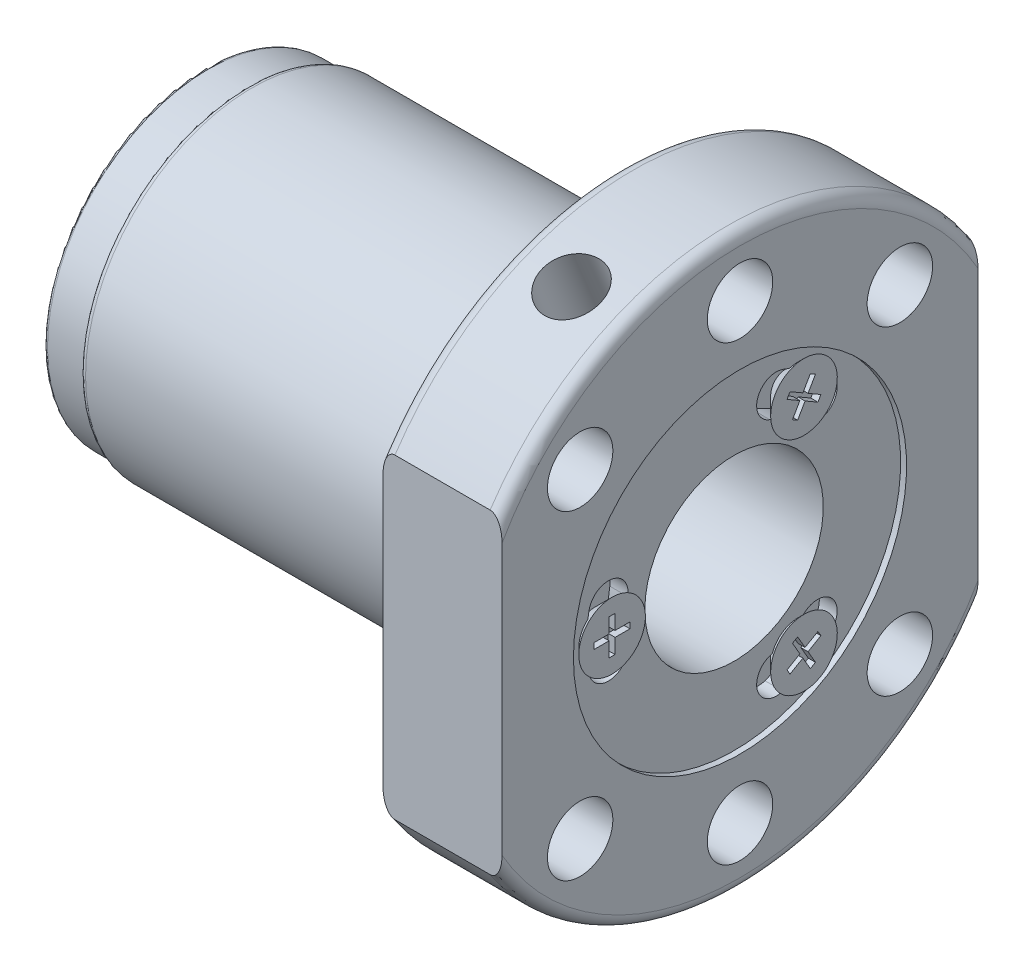
from build123d import *

# Parameters (mm, degrees)
SKETCH2_OUTSIDE_W   = 66.288
SKETCH2_OUTSIDE_H   = 66.288
SKETCH2_OUTSIDE_W_2 = 40
SKETCH2_OUTSIDE_H_2 = 48
CUT_EXTRUDE1_DEPTH  = 10
DIAMETERHOLE1_D     = 5.5
TAP1_REACH          = 66.874
TAP1_BORE_R         = 2.4585
CUT_EXTRUDE2_DEPTH  = 1.5
CUT_EXTRUDE3_DEPTH  = 0.6
CIRPATTERN1_COUNT   = 3


with BuildPart() as part:
    # Sketch1 → Revolve1 (revolve)
    with BuildSketch(Plane.XY, mode=Mode.PRIVATE) as revolve1_sk:
        with BuildLine():
            Line((10, 14), (9.5, 14))
            Line((9.5, 14), (9.5, 7.5))
            Line((9.5, 7.5), (-35, 7.5))
            Line((-35, 7.5), (-35, 13.2))
            ThreePointArc((-35, 13.2), (-34.912132034, 13.412132034), (-34.7, 13.5))
            Line((-34.7, 13.5), (-31.5, 13.5))
            ThreePointArc((-31.5, 13.5), (-31.353553391, 13.853553391), (-31, 14))
            Line((-31, 14), (0, 14))
            Line((0, 14), (0, 23))
            ThreePointArc((0, 23), (0.292893219, 23.707106781), (1, 24))
            Line((1, 24), (9, 24))
            ThreePointArc((9, 24), (9.707106781, 23.707106781), (10, 23))
            Line((10, 23), (10, 14))
        make_face()
    revolve(revolve1_sk.sketch.rotate(Axis((-37.257548112, 0, 0), (1, 0, 0)), 90), axis=Axis((-37.257548112, 0, 0), (1, 0, 0)))

    # Sketch2 outside → Cut-Extrude1 (cut)
    with BuildSketch(Plane(origin=(10, 0, 0), x_dir=(0, 0, -1), z_dir=(1, 0, 0))):
        Rectangle(SKETCH2_OUTSIDE_W, SKETCH2_OUTSIDE_H)
        Rectangle(SKETCH2_OUTSIDE_W_2, SKETCH2_OUTSIDE_H_2, mode=Mode.SUBTRACT)
    extrude(amount=-CUT_EXTRUDE1_DEPTH, mode=Mode.SUBTRACT)

    # DiameterHole1 (through all)
    with Locations(Plane(origin=(10, 0, 0), x_dir=(0, 0, -1), z_dir=(1, 0, 0))):
        with Locations((13.435028843, 13.435028843), (0, 19), (-13.435028843, 13.435028843), (-13.435028843, -13.435028843), (0, -19), (13.435028843, -13.435028843)):
            Hole(DIAMETERHOLE1_D / 2)

    # Tap1 bore → Tap1 (cut, up to next)
    with BuildSketch(Plane(origin=(0, 22.17310878, 9.184402377), x_dir=(1, 0, 0), z_dir=(0, 0.9238795325112865, 0.3826834323650906)), mode=Mode.PRIVATE) as tap1_sk1:
        with Locations((5, 0)):
            Circle(TAP1_BORE_R)
    tap1_tool1 = extrude(tap1_sk1.sketch, amount=-TAP1_REACH, mode=Mode.PRIVATE) & part.part
    add(tap1_tool1.solids().sort_by_distance((5, 22.173109, 9.184402))[0], mode=Mode.SUBTRACT)

    # Sketch7 → Cut-Extrude2 (cut)
    with BuildSketch(Plane(origin=(9.5, 0, 0), x_dir=(0, 0, -1), z_dir=(1, 0, 0))):
        with BuildLine():
            ThreePointArc((-12.183507635, 2.306976744), (-12.4, 0), (-12.183507635, -2.306976744))
            ThreePointArc((-12.183507635, -2.306976744), (-10.255338343, -3.621192548), (-8.941122539, -1.693023256))
            ThreePointArc((-8.941122539, -1.693023256), (-9.1, 0), (-8.941122539, 1.693023256))
            ThreePointArc((-8.941122539, 1.693023256), (-10.255338343, 3.621192548), (-12.183507635, 2.306976744))
        make_face()
        with BuildLine():
            ThreePointArc((8.089654284, 9.397738747), (6.2, 10.738715007), (4.093853351, 11.704715492))
            ThreePointArc((4.093853351, 11.704715492), (1.991624433, 10.691979804), (3.004360121, 8.589750885))
            ThreePointArc((3.004360121, 8.589750885), (4.55, 7.880831174), (5.936762418, 6.896727629))
            ThreePointArc((5.936762418, 6.896727629), (8.26371391, 7.070787255), (8.089654284, 9.397738747))
        make_face()
        with BuildLine():
            ThreePointArc((4.093853351, -11.704715492), (6.2, -10.738715007), (8.089654284, -9.397738747))
            ThreePointArc((8.089654284, -9.397738747), (8.26371391, -7.070787255), (5.936762418, -6.896727629))
            ThreePointArc((5.936762418, -6.896727629), (4.55, -7.880831174), (3.004360121, -8.589750885))
            ThreePointArc((3.004360121, -8.589750885), (1.991624433, -10.691979804), (4.093853351, -11.704715492))
        make_face()
    extrude(amount=-CUT_EXTRUDE2_DEPTH, mode=Mode.SUBTRACT)

    # Sketch8 → Revolve2 (revolve)
    with BuildSketch(Plane.XY.offset(10.75), mode=Mode.PRIVATE) as revolve2_sk:
        Polygon((8.5, 1.3), (10, 2.8), (10, 0), (8.5, 0), align=None)
    revolve2 = revolve(revolve2_sk.sketch.rotate(Axis((0, 0, 10.75), (1, 0, 0)), 180), axis=Axis((0, 0, 10.75), (1, 0, 0)))

    # Sketch9 → Cut-Extrude3 (cut)
    with BuildSketch(Plane(origin=(10, 0, 0), x_dir=(0, 0, -1), z_dir=(1, 0, 0))):
        Polygon((-12.25, 0.25), (-11, 0.25), (-11, 1.5), (-10.5, 1.5), (-10.5, 0.25), (-9.25, 0.25), (-9.25, -0.25), (-10.5, -0.25), (-10.5, -1.5), (-11, -1.5), (-11, -0.25), (-12.25, -0.25), align=None)
    cut_extrude3 = extrude(amount=-CUT_EXTRUDE3_DEPTH, mode=Mode.SUBTRACT)

    # CirPattern1: Revolve2, Cut-Extrude3 ×3 about axis
    cirpattern1_axis = Axis((0, 0, 0), (1, 0, 0))
    add([revolve2.rotate(cirpattern1_axis, i * 360 / CIRPATTERN1_COUNT) for i in range(1, CIRPATTERN1_COUNT)])
    add([cut_extrude3.rotate(cirpattern1_axis, i * 360 / CIRPATTERN1_COUNT) for i in range(1, CIRPATTERN1_COUNT)], mode=Mode.SUBTRACT)


solid = part.part
